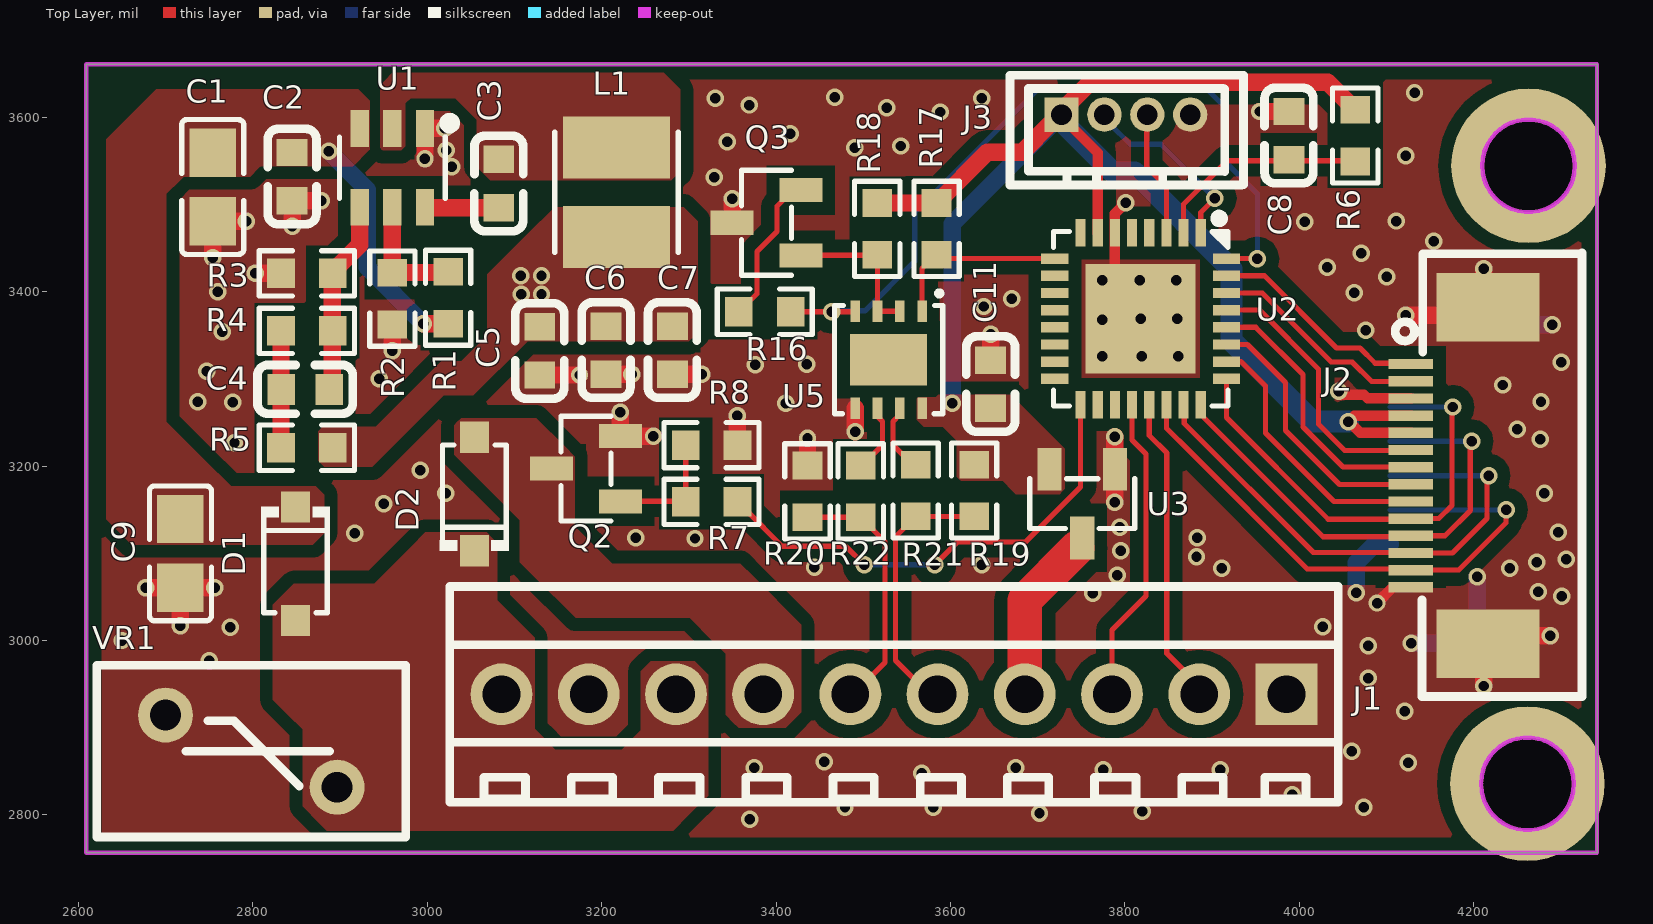
[diagram p0: Top Layer view]
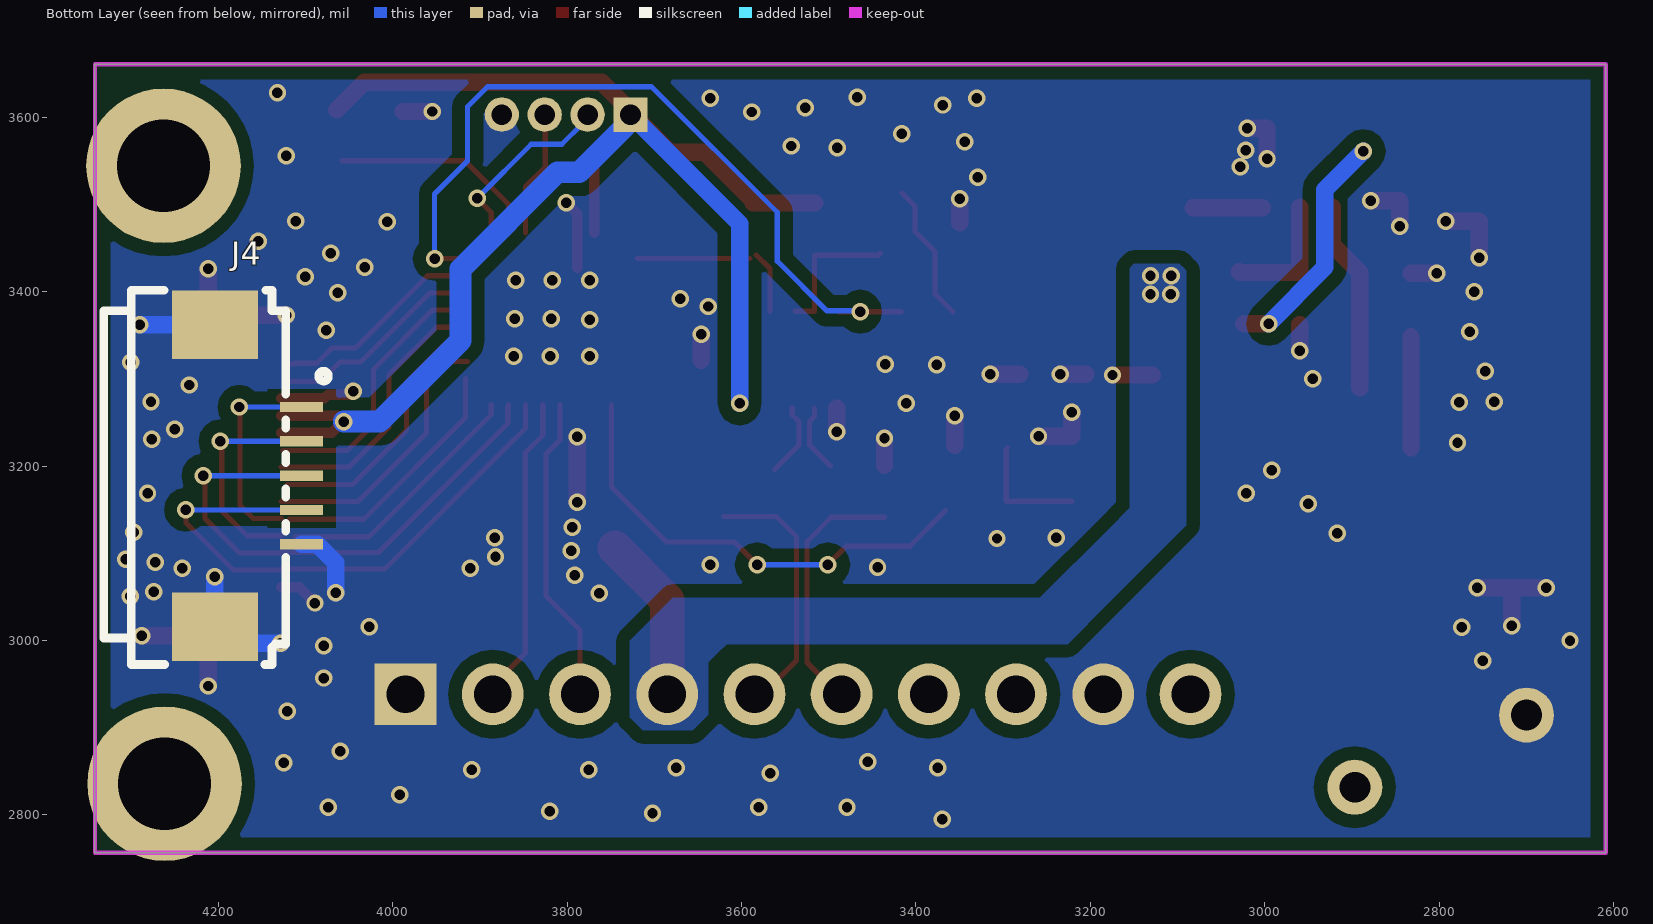
[diagram p1: Bottom Layer view, seen from below]
# Altium PCB MISC84392.PcbDoc
Units mil, origin at the board's own origin, x right, y up, seen from the top; angles counter-clockwise.
Board outline 1732.28 x 904.07 mil, 2 copper layers (Top Layer, Bottom Layer); 39 components, 36 nets, 154 pads, 145 vias.

## Layer stack, top to bottom (the 12.6 mil dielectric is the usual default, probably not edited)
Top Layer: signal copper 1.4
Dielectric: dielectric 12.6, FR-4, Dk 4.8
Bottom Layer: signal copper 1.4

## Board outline
2609.01,2756.7 4341.29,2756.7 4341.29,3660.77 2609.01,3660.77

## Design rules (kind name [scope] priority, off if disabled: settings)
Clearance Clearance_1 [inpolygon] p1: gap=6
Clearance [All] p2: gap=6
HoleSize [All] p1: absolutevalues=TRUE maxlimit=500 minlimit=1 maxpercent=80.000 minpercent=20.000
HoleToHoleClearance [All] p1: gap=0 allowstackedmicrovias=TRUE
MinimumSolderMaskSliver [All] p1: minsoldermaskwidth=0
PlaneClearance [All] p1: clearance=6
PlaneConnect [All] p1: planeconnectstyle=Direct reliefexpansion=20 reliefentries=4 reliefconductorwidth=10 reliefairgap=10
PolygonConnect [All] p1: connectstyle=Direct reliefconductorwidth=10 reliefentries=4 polygonreliefangle="90 Angle"
RoutingVias [All] p1: holewidth=12 width=20 viastyle="Through Hole" minholewidth=12 minwidth=20 maxholewidth=12 maxwidth=20
SilkToSilkClearance [All] p1: silktosilkclearance=0
SilkscreenOverComponentPads [All] p1: minsilkscreentomaskgap=0
SolderMaskExpansion [All] p1: expansion=4
Width [All] p1: maxlimit=40 minlimit=6 preferedwidth=6
21 further rules are at their usual default settings.

## Components (designator, comment, footprint, x,y, rotation, side; value= is the part's Value field where it differs from the comment)
C1 "10uF 35V" C0805 2754,3520 r270 top
C2 "0.1uf 50V" C0603 2845,3532 r90 top
C3 "0.1uf 50V" C0603 3082,3524 r270 top
C4 "75pf" C0603 2860,3288 r0 top
C5 "22uf 10V" C0603 3129,3332 r270 top
C6 "22uf 10V" C0603 3205,3333 r270 top
C7 "22uf 10V" C0603 3281,3333 r270 top
C8 "0.1uf 50V" C0603 3988,3579 r270 top
C9 "10uF 35V" C0805 2717,3100 r270 top
C11 "0.1uf 50V" C0603 3646,3294 r270 top
D1 "1N4148" SOD-123_L2.7-W1.7-LS3.8-RD 2849,3088 r270 top
D2 "1N4148" SOD-123_L2.7-W1.7-LS3.8-RD 3054,3168 r90 top
J1 "CONN-TH_DB125-2.54-10P-GN" CONN-TH_DB125-2.54-10P-GN 3535.13,2938.3 r180 top locked
J2 "AFC07-S14FCA-00" FPC-SMD_14P-P0.50_AFC07-S14FCA-00 4171.9,3189.17 r90 top locked
J3 "HC-1.25-4A" CONN-TH_4P-P1.25_HCTL_HC-1.25-4A 3801,3603 r0 top
J4 "AFA01-S05FCA-00" FPC-SMD_AFA01-S05FCA-00 4154,3189 r270 top
L1 "15uH" IND-SMD_L3.5-W3.0 3217,3514 r90 top
Q2 "AO3400" SOT-23-3_L2.9-W1.3-P1.90-LS2.4-BL-2 3182,3197 r90 top
Q3 "SS8050" SOT-23-3_L2.9-W1.3-P1.90-LS2.4-BR 3389,3479 r0 top
R1 "" R0603 3024,3393 r90 top
R2 "" R0603 2960,3392 r270 top
R3 "" R0603 2862,3421 r180 top
R4 "" R0603 2862,3355 r180 top
R5 "" R0603 2862,3221 r180 top
R6 "" R0603 4064,3579 r270 top
R7 "" R0603 3326,3159 r180 top
R8 "" R0603 3326,3224 r0 top
R16 "" R0603 3387,3377 r0 top
R17 "" R0603 3584,3472 r270 top
R18 "" R0603 3516,3472 r270 top
R19 "" R0603 3627,3172 r90 top
R20 "" R0603 3436,3171 r90 top
R21 "" R0603 3560,3172 r90 top
R22 "" R0603 3497,3171 r90 top
U1 "TPS54202DDCR" SOT-23-6_L2.9-W1.6-P0.95-LS2.8-BL 2960,3542 r180 top
U2 "QFN-32_L5.0-W5.0-P0.50-TL-EP3.1" QFN-32_L5.0-W5.0-P0.50-TL-EP3.1 3818,3369 r270 top
U3 "H7233-1" SOT-23-3_L2.9-W1.3-P1.90-LS2.4-BR 3751,3157 r90 top
U5 "SIT3088ETK" DFN-8_L3.0-W3.0-P0.65-BL-EP 3529,3322 r180 top
VR1 "RES-TH_L9.0-W5.0-P5.00-D0.8-S2.10" RES-TH_L9.0-W5.0-P5.00-D0.8-S2.10 2798.3,2873.14 r0 top locked

## Footprints (in the part's own frame and the unit in brackets; to place one, negate y for a bottom-side part, rotate by r counter-clockwise, add the part's x,y. Pads: shape width x height; smd on the part's side, far side on the other; paste and mask are expansions set on the pad)
C0603 [mm]
  rect 0.8x0.9 smd: 1(-0.7,0) 2(0.7,0)
  silkscreen extent -1.39,-0.71 1.39,0.71
C0805 [mm]
  rect 1.41x1.35 smd paste-100 mask+0.051: 1(-1,0) 2(1,0)
  silkscreen extent -1.96,-0.9 1.96,0.9
CONN-TH_4P-P1.25_HCTL_HC-1.25-4A [mm]
  rect 1x1 hole 0.6 paste+0 mask+0.05: 1(-1.875,0)
  round 1 hole 0.6 paste+0 mask+0.05: 2(-0.625,0) 3(0.625,0) 4(1.875,0)
  silkscreen extent -3.38,-2.06 3.43,1.15
CONN-TH_DB125-2.54-10P-GN [mm]
  rect 1.8x1.8 hole 1.1: 1(-11.43,0)
  round 1.8 hole 1.1: 2(-8.89,0) 3(-6.35,0) 4(-3.81,0) 5(-1.27,0) 6(1.27,0) 7(3.81,0) 8(6.35,0) 9(8.89,0) 10(11.43,0)
  silkscreen extent -12.94,-3.14 12.94,3.14
DFN-8_L3.0-W3.0-P0.65-BL-EP [mm]
  rect 0.28x0.625 smd: 1(-0.975,-1.412) 2(-0.325,-1.412) 3(0.325,-1.412) 4(0.975,-1.412) 5(0.975,1.412) 6(0.325,1.412) 7(-0.325,1.412) 8(-0.975,1.412)
  rect 2.25x1.5 smd: 9(0,0)
  silkscreen extent -1.58,-2.01 1.58,1.58
FPC-SMD_14P-P0.50_AFC07-S14FCA-00 [mm]
  rect 0.3x1.3 smd: 1(3.249,1.125) 2(2.745,1.125) 3(2.245,1.125) 4(1.745,1.125) 5(1.245,1.125) 6(0.745,1.125) 7(0.245,1.125) 8(-0.255,1.125) 9(-0.755,1.125) 10(-1.255,1.125) 11(-1.755,1.125) 12(-2.255,1.125) 13(-2.755,1.125) 14(-3.255,1.125)
  rect 2x3 smd: 15(-4.9,-1.125) 16(4.9,-1.125)
  silkscreen extent -6.44,-3.86 6.48,1.57
FPC-SMD_AFA01-S05FCA-00 [mm]
  rect 0.3x1.25 smd far side: 1(-2,-1.263) 2(-1,-1.263) 3(0,-1.263) 4(1,-1.263) 5(2,-1.263)
  rect 2x2.5 smd far side: 6(4.4,1.263) 7(-4.4,1.263)
IND-SMD_L3.5-W3.0 [mm]
  rect 1.8x3.12 smd: 1(1.303,0) 2(-1.303,0)
  silkscreen extent -1.75,-1.8 1.75,1.8
QFN-32_L5.0-W5.0-P0.50-TL-EP3.1 [mm]
  rect 0.8x0.3 smd paste-100 mask+0.051: 1(-2.5,1.75) 2(-2.5,1.25) 3(-2.5,0.75) 4(-2.5,0.25) 5(-2.5,-0.25) 6(-2.5,-0.75) 7(-2.5,-1.25) 8(-2.5,-1.75) 17(2.5,-1.75) 18(2.5,-1.25) 19(2.5,-0.75) 20(2.5,-0.25) 21(2.5,0.25) 22(2.5,0.75) 23(2.5,1.25) 24(2.5,1.75)
  rect 0.3x0.8 smd paste-100 mask+0.051: 9(-1.75,-2.5) 10(-1.25,-2.5) 11(-0.75,-2.5) 12(-0.25,-2.5) 13(0.25,-2.5) 14(0.75,-2.5) 15(1.25,-2.5) 16(1.75,-2.5) 25(1.75,2.5) 26(1.25,2.5) 27(0.75,2.5) 28(0.25,2.5) 29(-0.25,2.5) 30(-0.75,2.5) 31(-1.25,2.5) 32(-1.75,2.5)
  rect 3.2x3.2 smd paste-100 mask+0.051: 33(0,0)
  silkscreen extent -3.05,-2.54 2.54,2.54
R0603 [mil]
  rect 31.75x34.02 smd paste-3937.01 mask+2: 1(-29.66,0) 2(29.66,0)
  silkscreen extent -55,-26 55,26
RES-TH_L9.0-W5.0-P5.00-D0.8-S2.10 [mm]
  round 1.6 hole 0.9: 1(-2.5,1.05) 2(2.5,-1.05)
  silkscreen extent -4.5,-2.5 4.5,2.5
SOD-123_L2.7-W1.7-LS3.8-RD [mm]
  rect 0.91x0.84 smd: 1(-1.655,0) 2(1.655,0)
  silkscreen extent -1.65,-1 1.43,1
SOT-23-3_L2.9-W1.3-P1.90-LS2.4-BL-2 [mm]
  rect 0.7x1.25 smd: 1(-0.95,-1) 2(0.95,-1) 3(0,1)
  silkscreen extent -1.53,-0.73 1.53,0.73
SOT-23-3_L2.9-W1.3-P1.90-LS2.4-BR [mm]
  rect 1.25x0.7 smd: 1(1,-0.95) 2(1,0.95) 3(-1,0)
  silkscreen extent -0.73,-1.53 0.73,1.53
SOT-23-6_L2.9-W1.6-P0.95-LS2.8-BL [mil]
  rect 20.95x42.2 smd: 1(-37.4,-45.24) 2(0,-45.24) 3(37.4,-45.24) 4(37.4,45.24) 5(0,45.24) 6(-37.4,45.24)
  silkscreen extent -72,-57 61,35

## Part data
C1 C9: library part CL21A106KAYNNNE_C15850
C2 C3 C4 C5 C6 C7 C8 C11: library part CT41-0603-2F4-50V-0.1uF-M(N)
J1: library part DB125-2.54-10P-GN-S
L1: library part CMLF0302-150MTT
R1 R2 R3 R4 R5 R6 R7 R8 R16 R17 R18 R19 R20 R21 R22: library part RT0603BRD07105KL
U2: library part NCS25D34
VR1: library part FTR07D390K

## Free pads (board coordinates)
  round 177.17 hole 106.3: 0(4261.45,2835.73) 0(4262.69,3544.29)

## Via types
v1: diameter 20, hole 12, Top Layer to Bottom Layer, 145 vias

## Nets (pads, with @x,y where several pads share a name; then routed paths per layer and width w, separated by ;. In a path a pad name is that pad's centre, name@x,y a point inside that pad or via, vN(x,y) a via of type N, cw(c..) or ccw(c..) an arc to the next point about the centre after c; other vN are vias at no path point)
3.3V: C11.2 J2.4 J2.5 J3.1 R6.1 R17.1 R18.1 R19.2 U2.7 U3.2 U5.8 | length 1775.4
  Top Layer w12: J3.1@3739,3589 3768.79,3559.21 U2.7 ; v1(4056,3251) 4062.87,3257.87 J2.4 ; v1@4061,3247 4069.81,3238.19 J2.5
  Top Layer w20: R18.1 R17.1 ; R17.1@3586.66,3501.66 R17.1 ; J3.1@3716,3594 3682,3560 3642.34,3560 R17.1 ; J3.1@3731,3611 3760,3640 4032.66,3640 R6.1
  Bottom Layer w20: v1(3602,3272) 3602,3477.82 J3.1 ; J3.1@3731,3593 J3.1@3732.5,3591.5
  Bottom Layer w25: J3.1@3732,3591 3786,3537 3811,3537 3922,3426 3922,3344 4015,3251 v1(4056,3251)
+5V: C5.1 C6.1 C7.1 J1.4 L1.2 R5.1 U3.3 | length 192.5
  Top Layer w40: J1.4 3685.13,3046.13 U3.3@3745,3106
  other v1: 3108,3397 3131,3397 3107,3418 3131,3418
A1: J1.6 R20.1 R22.1 | length 272.1
  Top Layer w6: R20.1 R22.1 ; R22.1@3497.66,3141.34 R22.1 ; J1.6@3502,2952 3525,2975 3525,3113.34 R22.1
B1: J1.5 R19.1 R21.1 | length 286.1
  Top Layer w6: J1.5@3573,2941 3537,2977 3537,3119 3560,3142 R21.1 R19.1@3620.34,3142.34
BLK: J2.1 U2.31 | length 245.1
  Top Layer w6: U2.31 3959.79,3418.21 4042.5,3335.5 4069.5,3335.5 4087,3318 J2.1@4113,3318 ; J2.1@4113,3317 J2.1@4120,3317
CS: J2.2 U2.30 | length 245.6
  Top Layer w6: U2.30 3957.47,3398.53 4036.5,3319.5 4060.5,3319.5 4083,3297 J2.2@4120,3297
DC: J2.8 U2.27 | length 303.3
  Top Layer w6: U2.27 3940.53,3339.47 3984,3296 3984,3241 4046,3179 J2.8@4121,3179
GND: C1.2 C2.1 C5.2 C6.2 C7.2 C8.1 C9.2 C11.1 J1.1 J1.9 J2.3 J2.14 J2.15 J2.16 J3.4 J4.5 J4.6 J4.7 Q2.2 Q3.3 R2.2 R3.2 R8.2 R20.2 U1.1 U2.6 U2.33 U3.1 U5.5 VR1.1 | length 1615.8
  Top Layer w12: U2.33@3788.47,3427.53 U2.6 3788.47,3489.47 v1(3801,3502) ; v1(4045,3286) 4049,3282 v1@4052,3282 ; v1@4049,3285 v1@4052,3282 ; v1(4089,3043) 4107.02,3061.02 J2.14 ; J2.3 4078.44,3277.56 4074,3282 v1@4052,3282
  Top Layer w20: v1(2677.37,3060.63) C9.2 ; v1(2717,3017) C9.2 ; v1(2754,3439) C1.2 v1(2792.37,3480.63) ; v1(2756.37,3060.63) C9.2 ; v1(2803,3421) R3.2 ; v1(2845,3475) C2.1 v1(2878.44,3504.44) ; v1(2960,3332) R2.2 ; v1(2997.4,3552.4) U1.1 v1(3020.24,3587.24) ; C5.2 v1(3174.56,3304.44) ; C6.2 v1(3234.44,3305.44) ; v1(3221.37,3261.63) Q2.2 v1(3259.4,3234.4) ; C7.2 v1(3314.56,3305.44) ; Q3.3 v1(3349.63,3506.63) ; R8.2 v1(3355.66,3257.66) ; R20.2 v1(3436,3232) ; v1(3490.62,3239.38) U5.5 ; C11.1 v1(3646,3351) ; v1(3788.4,3158.4) U3.1 v1(3788.4,3233.6) ; v1(3954.44,3606.56) C8.1 ; v1(4122.03,3373.03) 4211.12,3373.03 v1(4211.12,3426.12) ; v1(4211.12,2947.88) 4211.12,3005.32 v1(4287.68,3005.32)
  Bottom Layer w20: v1(4065,3055) 4065,3089 4086.26,3110.26 J4.5 ; v1(4128,2997) 4184.93,2997 J4.6 4203.7,3072.7 v1(4204,3073) ; J4.7 v1(4289.77,3362.22)
  other v1: 3370,2795 3702,2802 3820,2804 3479,2809 3580,2809 4074,2809 3992,2823 3567,2848 3775,2852 3909,2852 3375,2854 3675,2854 4125,2860 3455,2861 4060,2873 4121,2919 4079,2957 2750,2977 4079,2994 2650,3000 2774,3015 4027,3016 4301,3051 3763,3054 4274,3056 3791,3075 3911,3083 4241,3083 3444,3084 3636,3087 4272,3090 4306,3093 3882,3096 3795,3103 3307,3117 3239,3118 3883,3118 2917,3123 4297,3124 3794,3130 2950,3157 3021,3169 4281,3169 2992,3195 2779,3227 4276,3231 4250,3242 3411,3272 2777,3273 2737,3274 4277,3274 4233,3293 2945,3300 2747,3309 3376,3316 3435,3317 4300,3319 3774,3326 3819,3326 3861,3326 2765,3354 4076,3356 3774,3368 3818,3369 3860,3369 3638,3383 3670,3392 4063,3399 2760,3400 3774,3413 3817,3413 3859,3413 4100,3417 4032,3428 4071,3444 4154,3458 4006,3480 4111,3481 3329,3531 3028,3543 4122,3556 3022,3562 3490,3565 3543,3567 3344,3572 3416,3581 3588,3606 3527,3611 3369,3614 3330,3622 3636,3622 3467,3623 4132,3628
NetC3_2: C3.2 U1.6 | length 79.4
  Top Layer w20: U1.6@3002.56,3496.44 C3.2
NetC4_1: C4.1 R4.2 R5.2 | length 127.3
  Top Layer w20: R5.2 R4.2@2832.34,3348.34
NetC4_2: C4.2 R3.1 R4.1 U1.4 | length 219.8
  Top Layer w20: C4.2@2891,3290 2891,3422 2922.6,3453.6 U1.4
NetQ2_1: Q2.1 R7.2 R8.1 | length 137
  Top Layer w6: Q2.1 3296.4,3159.6 3296.4,3219.6 R8.1@3295,3221
NetQ3_1: Q3.1 R18.2 U5.2 U5.3 | length 162.5
  Top Layer w6: Q3.1@3441,3444 3443.2,3441.8 3516.2,3441.8 U5.3 U5.2@3538.39,3377.61
NetQ3_2: Q3.2 R16.1 | length 160.3
  Top Layer w6: R16.1 3378,3397.66 3378,3446 3401,3469 3401,3498 Q3.2@3416,3513
NetR1_2: R1.2 R2.1 U1.5 | length 144.2
  Top Layer w20: U1.5 2960,3422 3028,3422 R1.2@3029,3423
NetR21_2: R21.2 U5.7 | length 85.2
  Top Layer w6: U5.7 3541.8,3258.8 3534,3251 3534,3224 R21.2@3562,3196
NetR22_2: R22.2 U5.6 | length 78.7
  Top Layer w6: R22.2@3498,3200 3522,3224 3522,3251 3516.2,3256.8 U5.6
PWM: R7.1 U2.17 | length 540.2
  Top Layer w6: R7.1@3366,3149 3407,3108 3480,3108 v1(3501,3087) ; v1(3582,3087) 3608,3113 3686,3113 3749.1,3176.1 U2.17
  Bottom Layer w6: v1(3501,3087) v1(3582,3087)
PWMO: D2.2 J1.7 Q2.3
RES: J2.9 U2.26 | length 326.4
  Top Layer w6: U2.26@3914,3320 3933,3320 3961,3292 3961,3238 4039.55,3159.45 J2.9 ; U2.26 U2.26@3931.11,3319.79
RST: C8.2 R6.2 U2.2 | length 244.2
  Top Layer w6: U2.2 3867.22,3500.22 3917,3550 R6.2@4058,3550
RX: J1.3 U2.20 | length 340.3
  Top Layer w6: J1.3@3785,2953 3785,3012 3824,3051 3824,3214 3808.16,3229.84 U2.20
RX1: R17.2 U2.9 U5.1 | length 200.3
  Top Layer w6: U5.1 3567.38,3426.38 R17.2@3583,3442 ; R17.2@3590.1,3437.9 U2.9
S1: J2.10 J4.1 U2.25 | length 555.1
  Top Layer w6: 3916.42,3271.42 3916.42,3294 ; U2.25 3916.42,3294 ; J2.10@4118,3139 4033,3139 3916.42,3255.58 3916.42,3294 ; J2.10 4159.76,3139.76 4175,3155 v1@4175,3268
  Bottom Layer w6: J4.1 v1(4175.74,3267.74)
S2: J2.11 J4.2 U2.24 | length 551.1
  Top Layer w6: U2.24 3886.9,3259.1 3911,3235 ; 3913,3233 3911,3235 ; J2.11@4112,3119 4027,3119 3911,3235 ; J2.11 4167.08,3120.08 4196,3149 v1@4196,3229
  Bottom Layer w6: J4.2 v1(4197.62,3228.38)
S3: J2.12 J4.3 U2.23 | length 608.4
  Top Layer w6: U2.23@3867.21,3267 U2.23 ; U2.23@3868,3267 3868,3249 4016,3101 J2.12@4128,3101 ; J2.12 4175.39,3100.39 4215,3140 v1@4215,3189
  Bottom Layer w6: J4.3 v1(4216.99,3189.01)
S4: J2.13 J4.4 U2.22 | length 648.7
  Top Layer w6: U2.22 3847.53,3243.47 3875,3216 4009,3082 J2.13@4127,3082 ; J2.13 4182.71,3080.71 4237,3135 v1(4237,3150)
  Bottom Layer w6: J4.4 v1@4232.64,3149.64
SCL: J2.6 U2.29 | length 313.1
  Top Layer w6: U2.29 3954.16,3378.84 4022,3311 4022,3248 4052,3218 J2.6@4126,3218
SDA: J2.7 U2.28 | length 313.1
  Top Layer w6: U2.28 3949.84,3359.16 4004,3305 4004,3245 4050,3199 J2.7@4128,3199
SW: C3.1 L1.1 U1.2
SWCLK: J3.3 U2.3 | length 137.9
  Top Layer w6: J3.3@3825,3596 3825,3543 3847.53,3520.47 U2.3
SWDIO: J3.2 U2.1 | length 201.5
  Top Layer w6: U2.1 3886.9,3490.9 v1(3903,3507)
  Bottom Layer w6: J3.2@3783,3592 3806,3569 3841,3569 3901,3509 v1(3903,3507)
TX: J1.2 U2.21 | length 347.7
  Top Layer w6: U2.21 3827.84,3235.16 3848,3215 3848,2985 J1.2@3886,2947
TX1: R16.2 U2.32 U5.4 | length 898.8
  Top Layer w6: R16.2 v1(3464,3377) U5.4@3488,3377 ; U2.32 v1(3951.9,3437.9)
  Bottom Layer w6: v1(3464,3377) v1@3468.5,3381.5 ; v1@3467,3378 3502,3378 3559,3435 3559,3491 3703,3635 3891,3635 3914,3612 3914,3550 3951.9,3512.1 v1(3951.9,3437.9)
VCC: D1.2 D2.1 J1.8 J1.10 VR1.2
VIN: C1.1 C2.2 C9.1 D1.1 R1.1 U1.3 | length 271
  Top Layer w20: v1(2995.66,3363.34) R1.1
  Bottom Layer w20: v1(2887,3561) 2931,3517 2931,3428 v1(2995.66,3363.34)
pads on no net: U2.4 U2.5 U2.8 U2.10 U2.11 U2.12 U2.13 U2.14 U2.15 U2.16 U2.18 U2.19 U5.9

## Polygon pours and split planes (outlines as drawn)
PWMO on Top Layer "Bottom Layer-No Net" (solid, remove dead copper, pour order 1000): 3031,3238 3031,3227 3031,3216 3031,3213 3092,3152 3106,3138 3106,3123 3106,3090 3121,3075 3170,3026 3237,3026 3301,3026 3327,3000 3342,2985 3342,2954 3342,2915 3351,2906 3357,2900 3379,2900 3411,2900 3419,2908 3429,2918 3429,2937 3429,3018 3373,3074 3359,3088 3305,3088 3212,3088 3192,3108 3169,3131 3169,3187 3169,3211 3158,3222 3125,3255 3074,3255 3039,3255 3034,3250 3031,3247 3031,3238
VCC on Top Layer "Bottom Layer-No Net" (solid, remove dead copper, pour order 1001): 2823,3032 2823,2932 2840,2915 2857,2898 2857,2860 2857,2810 2877,2790 2885,2782 2912,2782 3282,2782 3300,2800 3322,2822 3322,2934 3322,2961 3312,2971 3307,2976 3291,2976 3256,2976 3251,2971 3245,2965 3245,2946 3245,2897 3227,2879 3223,2875 3194,2875 3147,2875 3134,2888 3123,2899 3123,2932 3123,3003 3103,3023 3080,3046 3080,3087 3080,3112 3074,3118 3068,3124 3055,3124 2998,3124 2981,3107 2939,3065 2880,3065 2847,3065 2832,3050 2823,3041 2823,3032
3.3V on Top Layer "Bottom Layer-No Net" (solid, remove dead copper, pour order 1002): 3561,3266 3561,3253 3564,3250 3569,3245 3583,3245 3591,3245 3599,3237 3607,3229 3607,3212 3607,3188 3611,3184 3612,3183 3614,3183 3660,3183 3671,3172 3675,3168 3693,3168 3725,3168 3728,3171 3731,3174 3731,3176 3731,3220 3718,3233 3669,3282 3657,3282 3586,3282 3584,3280 3583,3279 3573,3279 3563,3279 3562,3278 3561,3277 3561,3266
VIN on Top Layer "Bottom Layer-No Net" (solid, remove dead copper, pour order 1003): 2632,3529 2632,3139 2652,3119 2661,3110 2703,3110 2869,3110 2877,3118 2882,3123 2882,3127 2882,3167 2876,3173 2872,3177 2848,3177 2775,3177 2744,3208 2701,3251 2701,3460 2701,3512 2717,3528 2721,3532 2740,3532 2797,3532 2807,3542 2809,3544 2831,3544 2915,3544 2933,3562 2934,3563 2934,3571 2934,3619 2929,3624 2921,3632 2908,3632 2689,3632 2649,3592 2632,3575 2632,3530
SW on Top Layer "Bottom Layer-No Net" (solid, remove dead copper, pour order 1004): 2946,3606 2946,3565 2948,3563 2949,3562 2955,3562 2970,3562 2972,3564 2975,3567 2975,3573 2975,3616 2981,3622 3012,3622 3032,3622 3039,3615 3057,3597 3057,3574 3057,3543 3064,3536 3072,3528 3165,3528 3280,3528 3284,3532 3290,3538 3290,3546 3290,3632 3278,3644 3271,3651 3196,3651 2960,3651 2951,3642 2946,3637 2946,3606
+5V on Top Layer "Bottom Layer-No Net" (solid, remove dead copper, pour order 1005): 2875,3228 2875,3206 2879,3202 2882,3199 2921,3199 2937,3199 3011,3273 3019,3281 3043,3281 3053,3281 3111,3339 3115,3343 3171,3343 3300,3343 3306,3349 3310,3353 3310,3358 3310,3481 3298,3493 3294,3497 3274,3497 3146,3497 3114,3465 3069,3420 3069,3394 3069,3350 3057,3338 3039,3320 3028,3320 3016,3320 2975,3279 2941,3245 2906,3245 2880,3245 2876,3241 2875,3240 2875,3228
GND on Top Layer "Bottom Layer-No Net" (solid, remove dead copper, pour order 1006): 2553.33,3548.29 2553.33,2759.29 2626.33,2686.29 2684.33,2628.29 2867.33,2628.29 4376.33,2628.29 4438.33,2690.29 4495.33,2747.29 4495.33,2866.29 4495.33,3690.29 4430.33,3755.29 4396.33,3789.29 4304.33,3789.29 2671.33,3789.29 2599.33,3717.29 2557.33,3675.29 2557.33,3552.29
+5V on Bottom Layer "Bottom Layer-No Net" (solid, remove dead copper, pour order 1007): 3090,3419 3090,3132 3188,3034 3218,3004 3226,2996 3587,2996 3617,2996 3627,2986 3638,2975 3638,2948 3638,2915 3646,2907 3656,2897 3687,2897 3713,2897 3722,2906 3728,2912 3728,2935 3728,3000 3687,3041 3679,3049 3621,3049 3258,3049 3178,3129 3155,3152 3155,3388 3155,3427 3152,3430 3150,3432 3140,3432 3098,3432 3092,3426 3090,3424 3090,3419
GND on Bottom Layer "Bottom Layer-No Net" (solid, remove dead copper, pour order 1008): 2552.51,3530 2552.51,2791 2613.51,2730 2686.51,2657 2904.51,2657 4353.51,2657 4414.51,2718 4449.51,2753 4449.51,2799 4449.51,3733 4410.51,3772 4360.51,3822 4249.51,3822 2672.51,3822 2606.51,3756 2556.51,3706 2556.51,3530

## Keep-outs
Top Layer:
  circle w5: c4262.69,3544.29 r53.15
  circle w5: c4261.45,2835.73 r53.15
Keep-Out Layer:
  the board outline again, w5